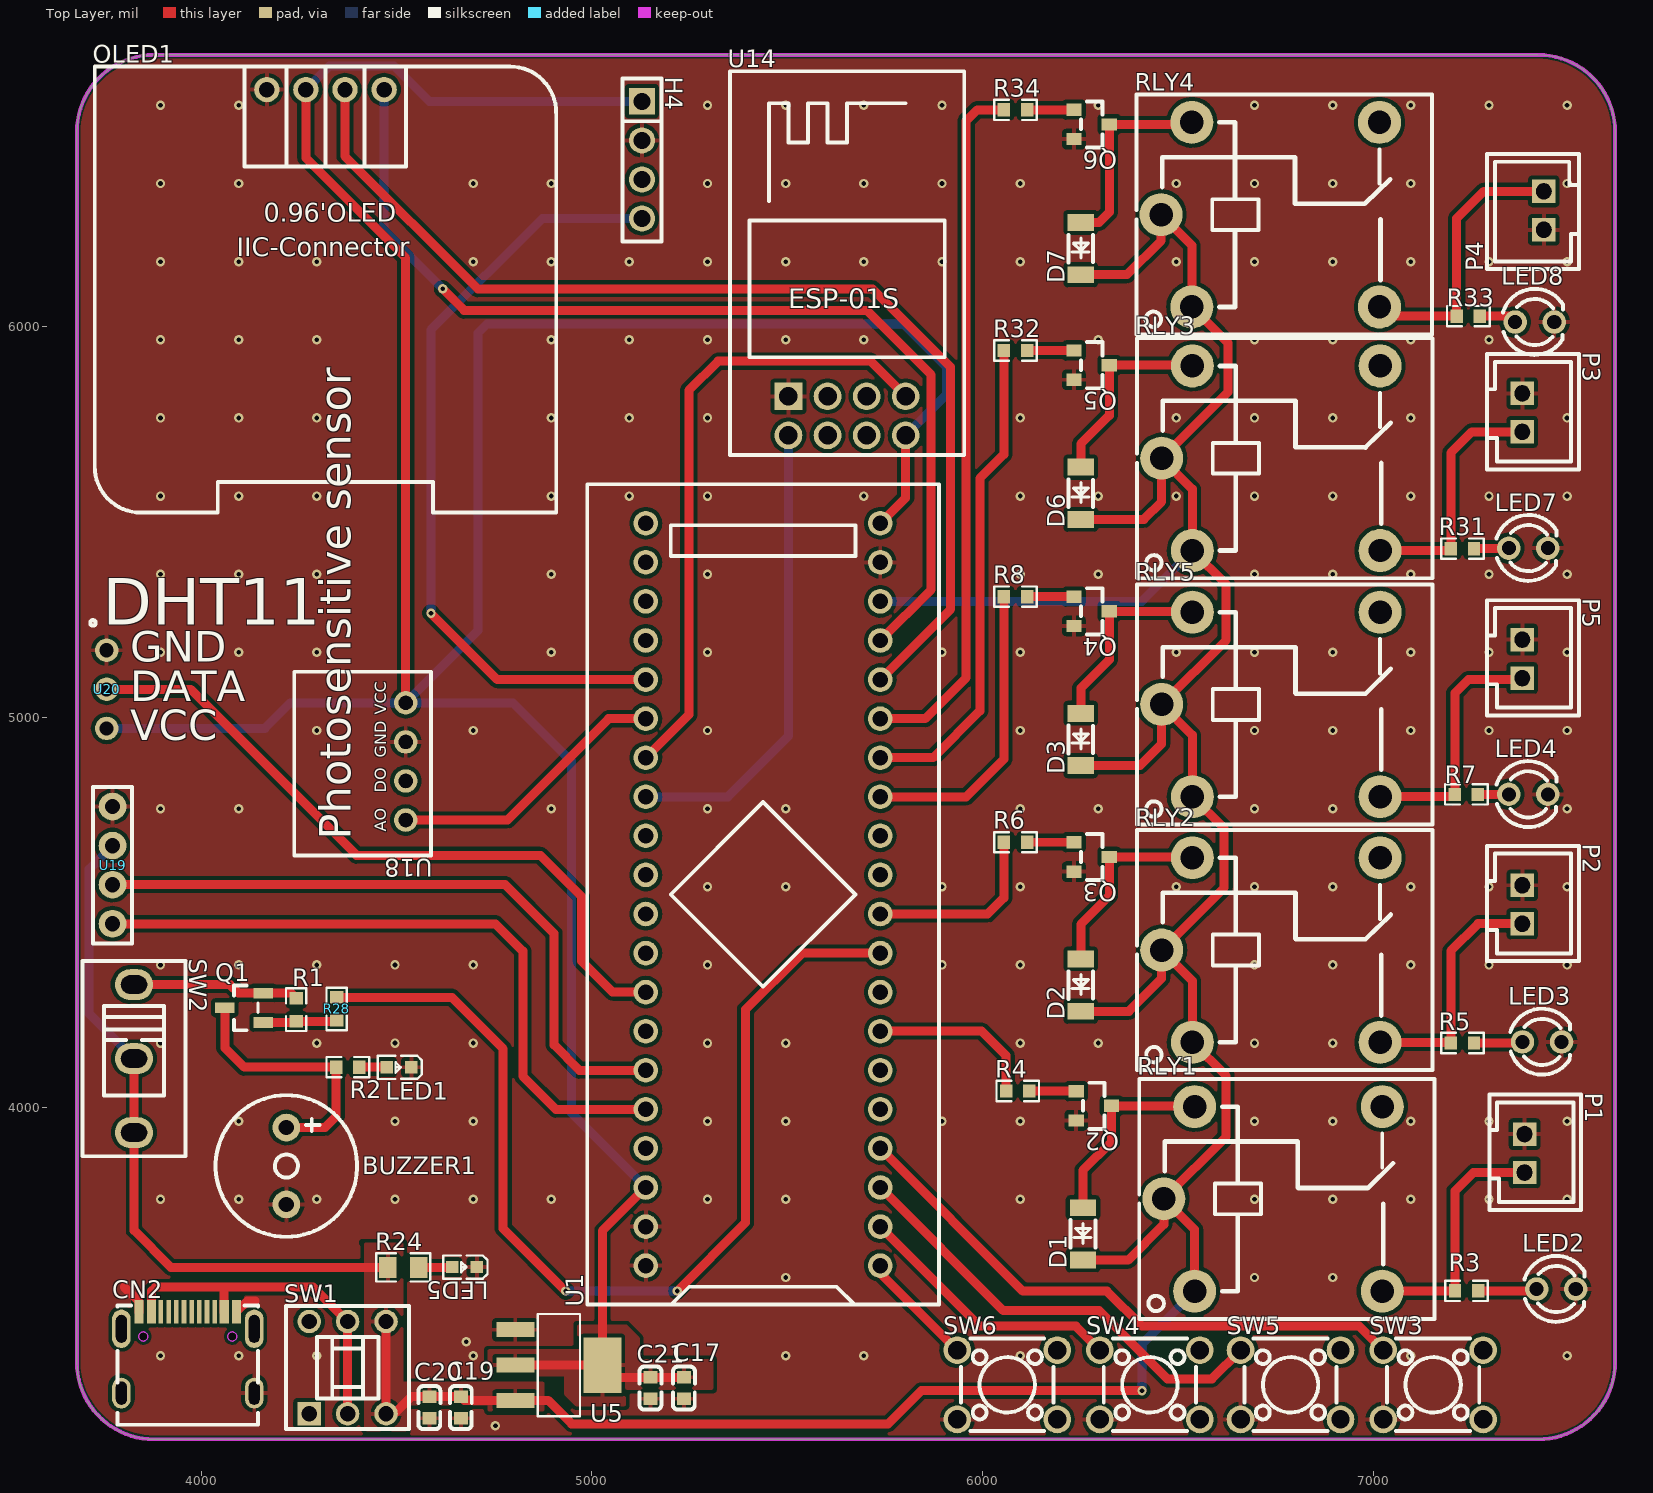
[diagram p0: Top Layer view]
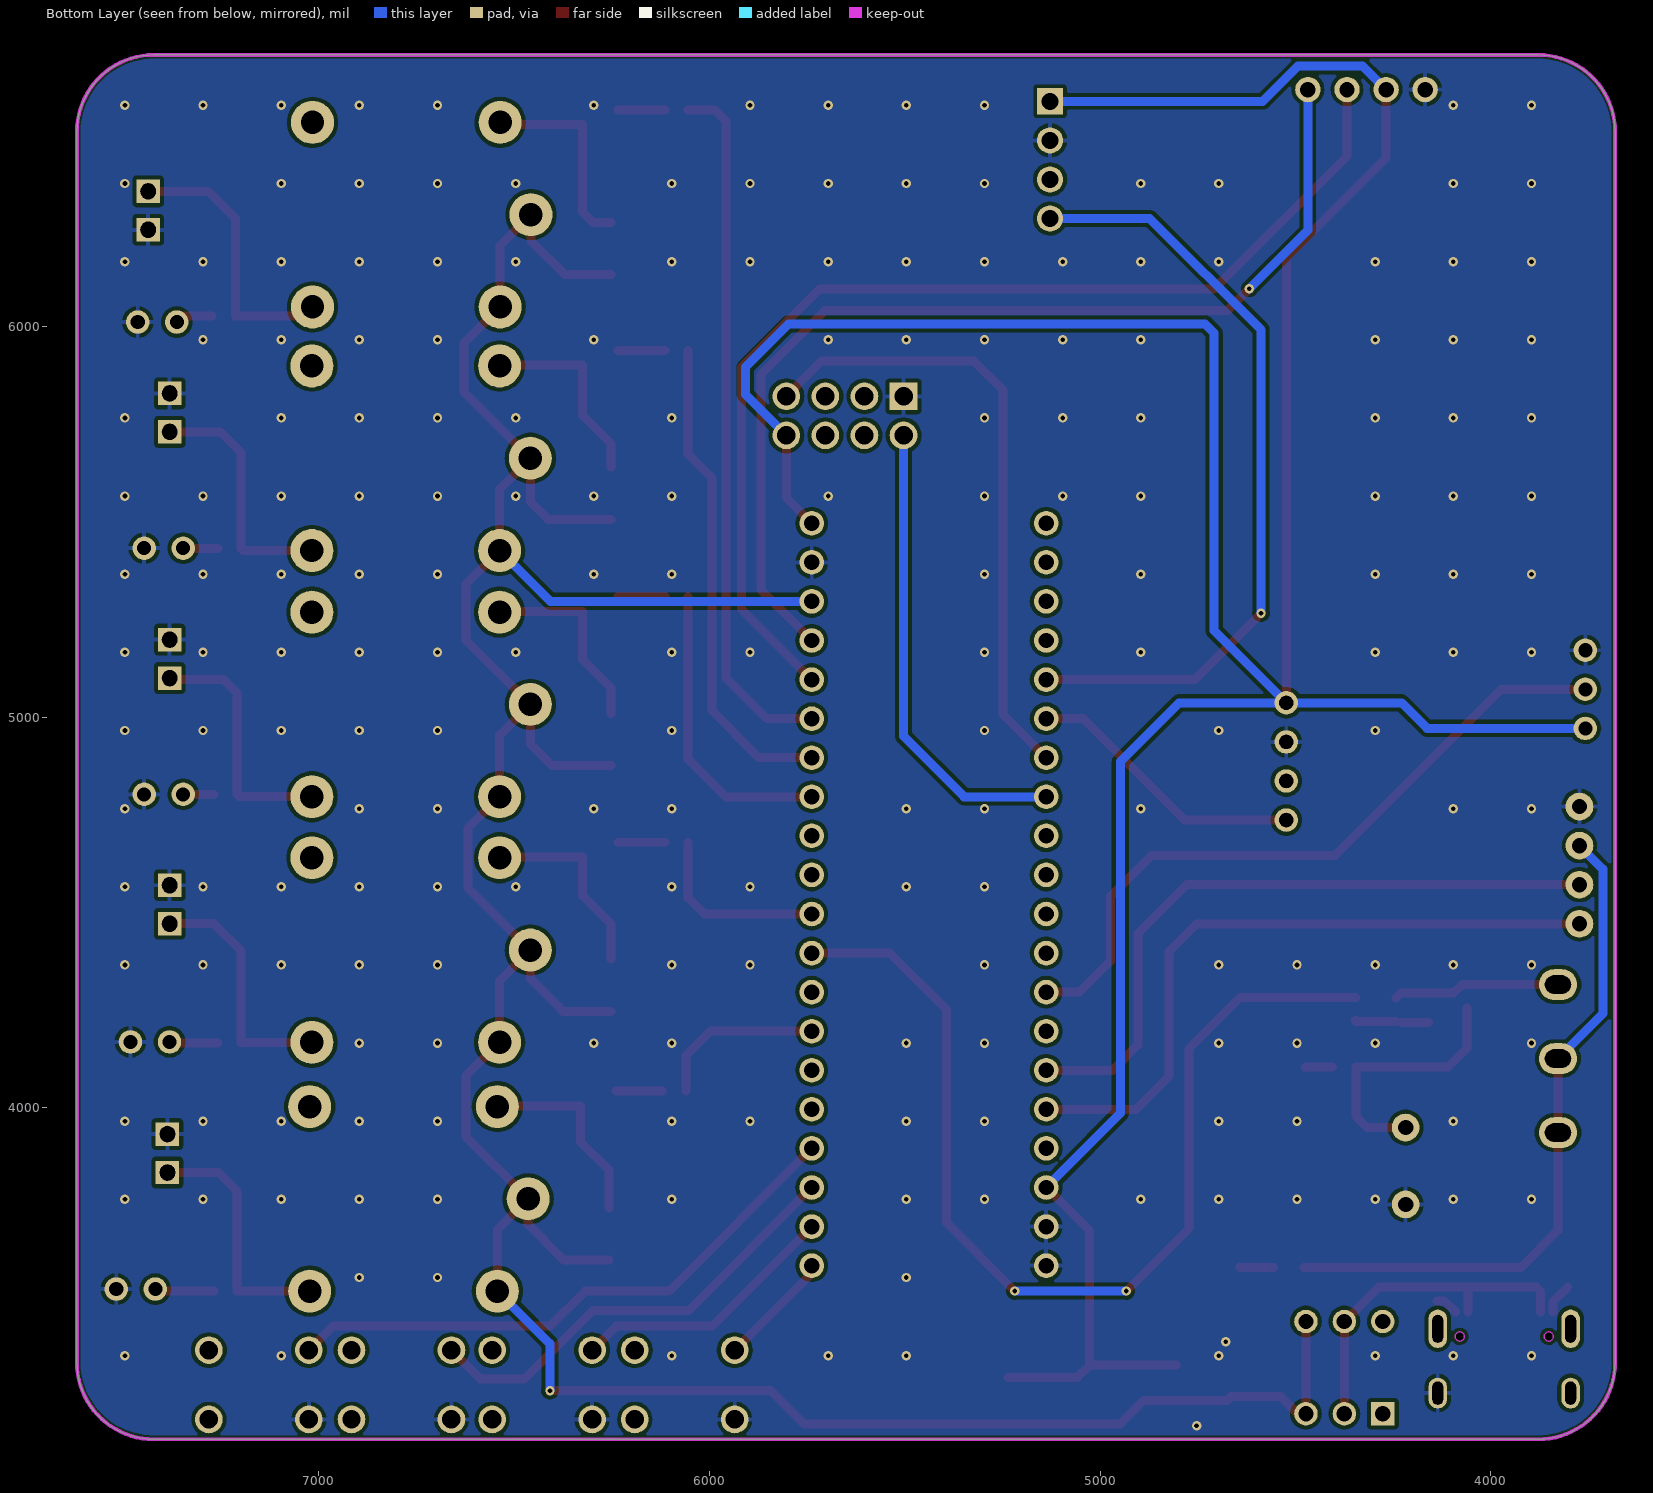
[diagram p1: Bottom Layer view, seen from below]
# Altium PCB MISC51965.pcbdoc
Units mil, origin at the board's own origin, x right, y up, seen from the top; angles counter-clockwise.
Board outline 3937.01 x 3543.31 mil, 2 copper layers (Top Layer, Bottom Layer), stack 62.206 mil thick; 62 components, 48 nets, 227 pads, 205 vias.

## Layer stack, top to bottom
Top Solder Mask Layer: solder mask 0.394, Dk 3.3
Top Layer: signal copper 1.379
Dielectric1: surface 59.449, FR4, Dk 4.5
Bottom Layer: signal copper 1.378
Bottom Solder Mask Layer: solder mask 0.394, Dk 3.3

## Board outline
3879.19,6694.72 ccw(c3879.19,6497.87) 3682.34,6497.87 3682.34,3348.26 ccw(c3879.19,3348.26) 3879.19,3151.41 7422.5,3151.41 ccw(c7422.5,3348.26) 7619.35,3348.26 7619.35,6497.87 ccw(c7422.5,6497.87) 7422.5,6694.72 3879.19,6694.72

## Design rules (kind name [scope] priority, off if disabled: settings)
BoardOutlineClearance copperThickness2oz_1 [All] p2 off: genericclearance=7.99 ignorepadtopadclearanceinfootprint=FALSE except(0: Arc-SplitContinuation Track-SplitContinuation SMDPad-SplitContinuation THPad-SplitContinuation Via-SplitContinuation Fill-SplitContinuation Region-SplitContinuation Poly-SplitContinuation Text-SplitContinuation Hole-SplitContinuation; 5.98: Arc-CutoutEdge SMDPad-CutoutEdge THPad-CutoutEdge Via-CutoutEdge Fill-CutoutEdge Region-CutoutEdge Text-CutoutEdge; 6.93: Hole-OutlineEdge Hole-CutoutEdge; 10: Poly-OutlineEdge Poly-CutoutEdge; 11.81: Arc-OutlineEdge Track-OutlineEdge SMDPad-OutlineEdge THPad-OutlineEdge Via-OutlineEdge Fill-OutlineEdge Region-OutlineEdge Text-OutlineEdge Track-CutoutEdge)
BoardOutlineClearance copperThickness1oz_1 [All] p4: genericclearance=4.02 ignorepadtopadclearanceinfootprint=FALSE except(0: Arc-SplitContinuation Track-SplitContinuation SMDPad-SplitContinuation THPad-SplitContinuation Via-SplitContinuation Fill-SplitContinuation Region-SplitContinuation Poly-SplitContinuation Text-SplitContinuation Hole-SplitContinuation; 6: SMDPad-CutoutEdge THPad-CutoutEdge Via-CutoutEdge Fill-CutoutEdge Region-CutoutEdge Text-CutoutEdge; 6.93: Hole-OutlineEdge Hole-CutoutEdge; 10: Poly-OutlineEdge Poly-CutoutEdge; 11.8: Arc-OutlineEdge Track-OutlineEdge SMDPad-OutlineEdge THPad-OutlineEdge Via-OutlineEdge Fill-OutlineEdge Region-OutlineEdge Text-OutlineEdge; 11.81: Arc-CutoutEdge Track-CutoutEdge)
Clearance copperThickness2oz [All] p1 off: gap=7.99 ignorepadtopadclearanceinfootprint=FALSE except(5.98: SMDPad-Track SMDPad-SMDPad THPad-Track SMDPad-THPad THPad-THPad Track-Via SMDPad-Via THPad-Via Via-Via Fill-Track Region-Track Fill-SMDPad Region-SMDPad Fill-THPad Region-THPad Fill-Via Region-Via Fill-Fill Fill-Region Region-Region Arc-Track Arc-SMDPad Arc-THPad Arc-Via Fill-Arc Region-Arc Arc-Arc Text-Track SMDPad-Text Text-THPad Text-Via Fill-Text Region-Text Arc-Text Text-Text; 6.93: Hole-Track Hole-SMDPad Hole-THPad Hole-Via Fill-Hole Region-Hole Hole-Arc Hole-Text; 10: Poly-Track Poly-SMDPad Poly-THPad Poly-Via Poly-Fill Poly-Region Poly-Poly Poly-Arc Poly-Text Poly-Hole)
Clearance copperThickness1oz [All] p3: gap=4.02 ignorepadtopadclearanceinfootprint=FALSE except(5.98: SMDPad-Track SMDPad-SMDPad THPad-Track SMDPad-THPad THPad-THPad Track-Via SMDPad-Via THPad-Via Via-Via Fill-Track Region-Track Fill-SMDPad Region-SMDPad Fill-THPad Region-THPad Fill-Via Region-Via Fill-Fill Fill-Region Region-Region; 6: Arc-Track Arc-SMDPad Arc-THPad Arc-Via Fill-Arc Region-Arc Arc-Arc Text-Track SMDPad-Text Text-THPad Text-Via Fill-Text Region-Text Arc-Text Text-Text; 6.93: Hole-Track Hole-SMDPad Hole-THPad Hole-Via Fill-Hole Region-Hole Hole-Arc Hole-Text; 10: Poly-Track Poly-SMDPad Poly-THPad Poly-Via Poly-Fill Poly-Region Poly-Poly Poly-Arc Poly-Text Poly-Hole)
DiffPairsRouting differentialPair [All] p1: maxlimit=6 minlimit=6 mostfreqgap=6 toplayer_minwidth=5 toplayer_prefwidth=10 toplayer_maxwidth=100 toplayer_mingap=6 toplayer_prefgap=6 toplayer_maxgap=6 bottomlayer_minwidth=5 bottomlayer_prefwidth=10 bottomlayer_maxwidth=100 bottomlayer_mingap=6 bottomlayer_prefgap=6 bottomlayer_maxgap=6 maxuncoupledlength=10
HoleToHoleClearance otherClearance [All] p1: gap=11.81 allowstackedmicrovias=TRUE
Length netLength [All] p1: minlimit=0 maxlimit=0
MatchedLengths netLengthTolerance [All] p1: tolerance=1000
PasteMaskExpansion pasteMaskExpansion [All] p1: expansion=0
PlaneConnect innerPlane [All] p1: planeconnectstyle=Relief reliefexpansion=20 reliefentries=4 reliefconductorwidth=10 reliefairgap=10
PolygonConnect copperRegion [All] p1: connectstyle=Relief reliefconductorwidth=10 reliefentries=4 polygonreliefangle="90 Angle" airgapwidth=10 via.connectstyle=Relief via.reliefconductorwidth=10 via.reliefentries=4 via.polygonreliefangle="90 Angle" via.airgapwidth=10
RoutingVias viaSize [All] p1: holewidth=12.01 width=24.02 viastyle="Through Hole" minholewidth=11.81 minwidth=19.68 maxholewidth=248.03 maxwidth=393.7
SolderMaskExpansion solderMaskExpansion [IsVia] p1: expansion=-1000 istentingtop=TRUE
SolderMaskExpansion solderMaskExpansion [All] p2: expansion=2 istentingtop=FALSE
Width copperThickness2oz_2 [All] p1 off: maxlimit=100 minlimit=8 preferedwidth=10
Width copperThickness1oz_2 [All] p2: maxlimit=100 minlimit=5 preferedwidth=10

## Components (designator, comment, footprint, x,y, rotation, side; value= is the part's Value field where it differs from the comment)
BUZZER1 "HNB09A03" BUZ-TH_BD9.0-P5.00-D0.6-FD 4218.56,3850.88 r270 top
C17 "100n" C0603 5236.12,3282.62 r90 top
C19 "100n" C0603 4665.04,3232.75 r90 top
C20 "10u" C0603 4584.63,3232.75 r90 top
C21 "22u" C0603 5150.42,3282.62 r90 top
CN2 "USB-TYPEC" USB-C-SMD_MC-307 3966.22,3373.55 r0 top
D1 "LL4148" LL-34_L3.5-W1.5-RD 6257.42,3676.99 r90 top
D2 "LL4148" LL-34_L3.5-W1.5-RD 6251.77,4313.8 r90 top
D3 "LL4148" LL-34_L3.5-W1.5-RD 6251.77,4942.46 r90 top
D6 "LL4148" LL-34_L3.5-W1.5-RD 6251.77,5572.56 r90 top
D7 "LL4148" LL-34_L3.5-W1.5-RD 6251.77,6198.97 r90 top
H4 "" HDR-TH_4P-P2.54-V-F 5128.56,6425.88 r270 top
LED1 "" LED_0603 4504.75,4103.27 r180 top
LED2 "" LED_TH-3mm 7468.56,3535.88 r0 top
LED3 "" LED_TH-3mm 7432.24,4168.48 r0 top
LED4 "" LED_TH-3mm 7397.24,4802.14 r0 top
LED5 "" LED_0603 4672.56,3592.05 r180 top
LED7 "" LED_TH-3mm 7397.24,5432.23 r0 top
LED8 "" LED_TH-3mm 7413.56,6010.88 r0 top
OLED1 "" 0.96OLED_4P 4318.56,6605.88 r0 top
P1 "XH2.54 straight socket 2P" CONN-TH_XH2.54-2P 7387.52,3883.4 r270 top
P2 "XH2.54 straight socket 2P" CONN-TH_XH2.54-2P 7381.88,4520.21 r270 top
P3 "XH2.54 straight socket 2P" CONN-TH_XH2.54-2P 7381.88,5778.97 r270 top
P4 "XH2.54 straight socket 2P" CONN-TH_XH2.54-2P 7436.88,6296.23 r90 top
P5 "XH2.54 straight socket 2P" CONN-TH_XH2.54-2P 7381.88,5148.87 r270 top
Q1 "" S8550P_SOT 4108.56,4255.88 r0 top
Q2 "" S8050_SOT-23 6285.17,4009.98 r180 top
Q3 "" S8050_SOT-23 6279.53,4646.79 r180 top
Q4 "" S8050_SOT-23 6279.53,5275.45 r180 top
Q5 "" S8050_SOT-23 6279.53,5905.55 r180 top
Q6 "" S8050_SOT-23 6279.53,6521.7 r180 top
R1 "10k" R0603 4243.56,4250.88 r270 top
R2 "1k" R0603 4375.75,4103.67 r180 top
R3 "3.3k" R0603 7239.24,3531.48 r0 top
R4 "1k" R0603 6090.38,4042.7 r0 top
R5 "3.3k" R0603 7228.56,4165.88 r0 top
R6 "1k" R0603 6084.73,4679.51 r0 top
R7 "3.3k" R0603 7238.6,4801.95 r0 top
R8 "1k" R0603 6084.73,5308.17 r0 top
R24 "4.7k" R0805 4517.71,3591.37 r0 top
R28 "1k" R0603 4347.14,4252.97 r270 top
R31 "3.3k" R0603 7228.56,5430.88 r0 top
R32 "1k" R0603 6084.73,5938.26 r0 top
R33 "3.3k" R0603 7243.56,6025.88 r0 top
R34 "1k" R0603 6084.73,6554.14 r0 top
RLY1 "SRD-05VDC-SL-C" RELAY-TH_SRD-XXVDC-XL-C 6743.86,3766.8 r0 top
RLY2 "SRD-05VDC-SL-C" RELAY-TH_SRD-XXVDC-XL-C 6738.22,4403.6 r0 top
RLY3 "SRD-05VDC-SL-C" RELAY-TH_SRD-XXVDC-XL-C 6738.22,5662.36 r0 top
RLY4 "SRD-05VDC-SL-C" RELAY-TH_SRD-XXVDC-XL-C 6736.75,6285.76 r0 top
RLY5 "SRD-05VDC-SL-C" RELAY-TH_SRD-XXVDC-XL-C 6738.22,5032.27 r0 top
SW1 "K8-8081D-NNW" SW-TH_6P-L8.0-W8.0-P2.50 4375.18,3334.76 r0 top
SW2 "XY-SS12D10L3" SW-TH_3P-L12.7-W6.7_XY-SS12D10LXX 3828.56,4125.88 r270 top
SW3 "" SW-TH_4P-L6.0-W6.0-P4.50-LS6.5 7153.56,3290.88 r0 top
SW4 "" SW-TH_4P-L6.0-W6.0-P4.50-LS6.5 6428.56,3290.88 r0 top
SW5 "" SW-TH_4P-L6.0-W6.0-P4.50-LS6.5 6788.56,3290.88 r0 top
SW6 "" SW-TH_4P-L6.0-W6.0-P4.50-LS6.5 6063.56,3290.88 r0 top
U1 "LCKFB-DKX-STM32F103C8T6" CONN-TH_L53.3-W22.9_STM32F103C8T6-CARD 5438.56,4545.88 r90 top
U5 "TLV1117LV33DCYT" SOT-223-4_L6.5-W3.5-P2.30-LS7.0-BR 4915.99,3341.32 r180 top
U14 "ESP-01S" WIFIM-TH_ESP-01S 5653.56,5770.88 r0 top
U18 "Light intensity module" 光敏传感器 4498.56,4870.88 r180 top
U19 "" 4P排母 3723.56,4820.88 r270 top
U20 "" dht11温湿度传感器 3758.56,5170.88 r0 top

## Footprints (in the part's own frame and the unit in brackets; to place one, negate y for a bottom-side part, rotate by r counter-clockwise, add the part's x,y. Pads: shape width x height; smd on the part's side, far side on the other; paste and mask are expansions set on the pad)
0.96OLED_4P [mm]
  round 1.65 hole 1 copper offset 0,0: 1(-3.81,-0.001) 2(-1.27,0.002) 3(1.27,0.002) 4(3.81,0.002)
  silkscreen extent -15,-27.5 15,1.5
4P排母 [mm]
  round 1.8 hole 1: 1(1.27,1.27) 2(3.81,1.27) 3(6.35,1.27) 4(8.89,1.27)
  silkscreen extent 0,0 10.16,2.54
BUZ-TH_BD9.0-P5.00-D0.6-FD [mm]
  round 1.8 hole 1 copper offset 0,0 paste+0 mask+0.051: 1(-2.5,0) 2(2.5,0)
  silkscreen extent -4.6,-4.6 4.6,4.6
C0603 [mm]
  rect 0.8x0.9 smd paste+0 mask+0.051: 1(-0.7,0) 2(0.7,0)
  silkscreen extent -1.41,-0.71 1.39,0.72
CONN-TH_L53.3-W22.9_STM32F103C8T6-CARD [mm]
  round 1.6 hole 1: 1(-24.13,-7.62) 2(-21.59,-7.62) 3(-19.05,-7.62) 4(-16.51,-7.62) 5(-13.97,-7.62) 6(-11.43,-7.62) 7(-8.89,-7.62) 8(-6.35,-7.62) 9(-3.81,-7.62) 10(-1.27,-7.62) 11(1.27,-7.62) 12(3.81,-7.62) 13(6.35,-7.62) 14(8.89,-7.62) 15(11.43,-7.62) 16(13.97,-7.62) 17(16.51,-7.62) 18(19.05,-7.62) 19(21.59,-7.62) 20(24.13,-7.62) 21(24.13,7.62) 22(21.59,7.62) 23(19.05,7.62) 24(16.51,7.62) 25(13.97,7.62) 26(11.43,7.62) 27(8.89,7.62) 28(6.35,7.62) 29(3.81,7.62) 30(1.27,7.62) 31(-1.27,7.62) 32(-3.81,7.62) 33(-6.35,7.62) 34(-8.89,7.62) 35(-11.43,7.62) 36(-13.97,7.62) 37(-16.51,7.62) 38(-19.05,7.62) 39(-21.59,7.62) 40(-24.13,7.62)
  silkscreen extent -26.67,-11.43 26.67,11.43
CONN-TH_XH2.54-2P [mil]
  rect 60x60 hole 39.37 slot 41.34 at 0 deg paste+0 mask+1.97: 1(-49.22,0) 2(49.21,0)
  silkscreen extent -150,-90 145,145
dht11温湿度传感器 [mil]
  round 60 hole 36: 1(0,0) 2(0,-100) 3(0,-200)
  silkscreen extent -42,63 -28,77
HDR-TH_4P-P2.54-V-F [mm]
  rect 1.7x1.7 hole 1.1: 1(-3.81,0)
  round 1.7 hole 1.1: 2(-1.27,0) 3(1.27,0) 4(3.81,0)
  silkscreen extent -5.29,-1.27 5.29,1.27
LED_0603 [mil]
  rect 31.5x31.5 smd paste+0 mask+2: 1(-33.5,-0.4) 2(29.5,-0.2)
  silkscreen extent -61,-30 53,30
LED_TH-3mm [mil]
  round 60 hole 36 paste+0 mask+2: 1(-50,0) 2(50,0)
  silkscreen extent -81,-84 72,85
LL-34_L3.5-W1.5-RD [mm]
  rect 1.1x1.7 smd paste+0 mask+0.051: 1(-1.7,0) 2(1.7,0)
  silkscreen extent -0.9,-0.8 0.9,0.8
R0603 [mil]
  rect 31.75x34.02 smd paste-3937.01 mask+2: 1(-29.65,0) 2(29.66,0)
  silkscreen extent -55,-26 55,26
R0805 [mm]
  rect 1.133x1.377 smd paste-100 mask+0.051: 1(-1,0) 2(1,0)
  silkscreen extent -1.76,-0.92 1.76,0.92
RELAY-TH_SRD-XXVDC-XL-C [mil]
  round 110 hole 60: 1(-200.79,-236.22) 2(279.53,-236.2) 3(279.53,236.2) 4(-200.79,236.22) 5(-279.53,0)
  silkscreen extent -342,-307 413,307
S8050_SOT-23 [mm]
  rect 1x0.8 smd paste+0 mask+0.051: 1(1.15,-0.823) 2(1.15,1.077) 3(-1.15,0.127)
  silkscreen extent -0.7,-1.37 0.7,1.63
S8550P_SOT [mil]
  rect 49.2x27.6 smd paste+0 mask+2: 1(50.84,-37.4) 2(50.84,37.4) 3(-47.56,0)
  silkscreen extent -24,-58 37,58
SOT-223-4_L6.5-W3.5-P2.30-LS7.0-BR [mm]
  rect 2.47x0.98 smd paste+0 mask+0.051: 1(2.835,-2.3) 2(2.835,0) 3(2.835,2.3)
  rect 2.47x3.6 smd paste+0 mask+0.051: 4(-2.835,0)
  silkscreen extent -1.37,-3.33 1.37,3.33
SW-TH_3P-L12.7-W6.7_XY-SS12D10LXX [mm]
  oval 2x2.5 hole 1.2 slot 1.7 at 90 deg: 1(-4.81,0) 2(0,0) 3(4.81,0)
  silkscreen extent -6.35,-3.35 6.35,3.35
SW-TH_4P-L6.0-W6.0-P4.50-LS6.5 [mm]
  round 1.8 hole 1.2: 1(-3.25,2.25) 2(3.25,2.25) 3(-3.25,-2.25) 4(3.25,-2.25)
  silkscreen extent -3,-3 3,3
SW-TH_6P-L8.0-W8.0-P2.50 [mil]
  rect 60x60 hole 39.37 paste+0 mask+2: 1(-98.43,-118.11)
  round 60 hole 39.37 paste+0 mask+2: 2(0,-118.11) 3(98.42,-118.11) 4(-98.43,118.11) 5(0,118.11) 6(98.42,118.11)
  silkscreen extent -157,-157 157,157
USB-C-SMD_MC-307 [mm]
  oval 1.2x2 hole 0.7 slot 1.5 at 90 deg paste+0 mask+0.051: 0(4.32,-2.64) 1(-4.32,-2.64)
  oval 1.2x2.5 hole 0.7 slot 1.8 at 90 deg paste+0 mask+0.051: 2(4.32,1.54) 3(-4.32,1.54)
  rect 0.6x1.524 smd paste-100 mask+0.051: A1B12(-3.165,2.64) A4B9(-2.365,2.64) B1A12(3.165,2.64) B4A9(2.365,2.64)
  rect 0.3x1.524 smd paste-100 mask+0.051: A5(-1.25,2.64) A6(-0.25,2.64) A7(0.25,2.64) A8(1.25,2.64) B5(1.75,2.64) B6(0.75,2.64) B7(-0.75,2.64) B8(-1.75,2.64)
  Board Outline Layer circle w0.003: c-2.89,1.04 r0.3
  Board Outline Layer circle w0.003: c2.89,1.04 r0.3
  Board Outline Layer region: -2.59,1.04 -2.62,0.91 -2.703,0.806 -2.823,0.748 -2.957,0.748 -3.077,0.806 -3.16,0.91 -3.19,1.04 -3.19,1.04 -3.16,1.17 -3.077,1.275 -2.957,1.333 -2.823,1.333 -2.703,1.275 -2.62,1.17 -2.59,1.04
  Board Outline Layer region: -2.59,1.04 -2.599,0.968 -2.624,0.901 -2.665,0.841 -2.72,0.793 -2.784,0.76 -2.854,0.742 -2.926,0.742 -2.996,0.76 -3.06,0.793 -3.115,0.841 -3.156,0.901 -3.181,0.968 -3.19,1.04 -3.181,1.112 -3.156,1.18 -3.115,1.239 -3.06,1.287 -2.996,1.321 -2.926,1.338 -2.854,1.338 -2.784,1.321 -2.72,1.287 -2.665,1.239 -2.624,1.18 -2.599,1.112
  Board Outline Layer region: 3.19,1.04 3.16,0.91 3.077,0.806 2.957,0.748 2.823,0.748 2.703,0.806 2.62,0.91 2.59,1.04 2.59,1.04 2.62,1.17 2.703,1.275 2.823,1.333 2.957,1.333 3.077,1.275 3.16,1.17 3.19,1.04
  Board Outline Layer region: 3.19,1.04 3.181,0.968 3.156,0.901 3.115,0.841 3.06,0.793 2.996,0.76 2.926,0.742 2.854,0.742 2.784,0.76 2.72,0.793 2.665,0.841 2.624,0.901 2.599,0.968 2.59,1.04 2.599,1.112 2.624,1.18 2.665,1.239 2.72,1.287 2.784,1.321 2.854,1.338 2.926,1.338 2.996,1.321 3.06,1.287 3.115,1.239 3.156,1.18 3.181,1.112
  Multi-Layer board cut-out: -2.59,1.04 -2.62,0.91 -2.703,0.806 -2.823,0.748 -2.957,0.748 -3.077,0.806 -3.16,0.91 -3.19,1.04 -3.19,1.04 -3.16,1.17 -3.077,1.275 -2.957,1.333 -2.823,1.333 -2.703,1.275 -2.62,1.17 -2.59,1.04
  Multi-Layer board cut-out: 3.19,1.04 3.16,0.91 3.077,0.806 2.957,0.748 2.823,0.748 2.703,0.806 2.62,0.91 2.59,1.04 2.59,1.04 2.62,1.17 2.703,1.275 2.823,1.333 2.957,1.333 3.077,1.275 3.16,1.17 3.19,1.04
  silkscreen extent -4.57,-4.7 4.57,3.05
WIFIM-TH_ESP-01S [mm]
  rect 1.8x1.8 hole 1.2: 1(-3.81,1.27)
  round 1.8 hole 1.2: 2(-1.27,1.27) 3(1.27,1.27) 4(3.81,1.27) 5(3.81,-1.27) 6(1.27,-1.27) 7(-1.27,-1.27) 8(-3.81,-1.27)
  silkscreen extent -7.62,-2.54 7.62,22.4
光敏传感器 [mil]
  round 60 hole 36 slot 36.2 at 90 deg: 1(-25.45,-165.45) 2(-25.45,-65.45) 3(-25.45,34.55) 4(-25.45,134.55)
  silkscreen extent -90,-245 260,225

## Via types
v1: diameter 24.02, hole 12, Top Layer to Bottom Layer, 205 vias

## Nets (pads, with @x,y where several pads share a name; then routed paths per layer and width w, separated by ;. In a path a pad name is that pad's centre, name@x,y a point inside that pad or via, vN(x,y) a via of type N, cw(c..) or ccw(c..) an arc to the next point about the centre after c; other vN are vias at no path point)
$1N25: Q6.1 R34.2 | length 119.8
  Top Layer w23: R34.2 Q6.1@6234.21,6554.14
$1N27: D7.2 Q6.3 RLY4.4 | length 521.8
  Top Layer w23: D7.2 6298.58,6265.9 6324.8,6292.12 Q6.3 6530.68,6516.7 RLY4.4
$1N29: P4.2 R33.1 RLY4.2 | length 709.4
  Top Layer w23: RLY4.2 7039.96,6025.88 R33.1 7213.9,6276.22 7283.13,6345.45 P4.2
$1N33: LED8.1 R33.2 | length 96.6
  Top Layer w23: R33.2 7348.56,6025.88 LED8.1
$1N35: Q5.1 R32.2 | length 120
  Top Layer w23: R32.2 6233.94,5938.26 Q5.1
$1N37: D6.2 Q5.3 RLY3.4 | length 504.7
  Top Layer w23: D6.2 6251.77,5699.09 6324.8,5772.12 Q5.3 6535.46,5900.54 RLY3.4
$1N39: P3.2 R31.1 RLY3.2 | length 633.6
  Top Layer w23: RLY3.2 7194.18,5426.16 R31.1 7198.9,5676.22 7252.43,5729.75 P3.2
$1N43: LED7.1 R31.2 | length 89.6
  Top Layer w23: R31.2 7345.89,5430.88 LED7.1
$1N57: LED5.2 R24.2 | length 86.3
  Top Layer w23: R24.2 4642.18,3591.37 LED5.2
$1N74: BUZZER1.1 Q1.3 R2.2 | length 673
  Top Layer w23: Q1.3 4061,4153.44 4110.77,4103.67 R2.2 4346.09,3978.41 4316.98,3949.3 BUZZER1.1
$1N76: Q1.1 R1.2 R28.2 | length 173.6
  Top Layer w23: Q1.1 R1.2@4228.56,4218.48 ; R1.2 4345.05,4221.22 R28.2
$1N136: Q1.2 R1.1 SW2.1 | length 429.4
  Top Layer w23: SW2.1@3828.56,4315.25 4074.19,4315.25 4096.16,4293.28 Q1.2 4230.81,4293.28 R1.1
$1N137: LED1.2 R2.1 | length 69.9
  Top Layer w23: R2.1 4475.05,4103.67 LED1.2
$1N147: Q2.1 R4.2 | length 120
  Top Layer w23: R4.2 6239.58,4042.7 Q2.1
$1N149: D1.2 Q2.3 RLY1.4 | length 504.7
  Top Layer w23: D1.2 6257.42,3839.74 6330.45,3912.77 Q2.3 6541.11,4004.98 RLY1.4
$1N151: P1.2 R3.1 RLY1.2 | length 639.5
  Top Layer w23: RLY1.2 7208.7,3530.6 R3.1 7209.58,3786.9 7256.87,3834.19 P1.2
$1N155: LED2.1 R3.2 | length 151.5
  Top Layer w23: R3.2 7414.16,3531.48 LED2.1
$1N157: Q3.1 R6.2 | length 120
  Top Layer w23: R6.2 6233.94,4679.51 Q3.1
$1N159: D2.2 Q3.3 RLY2.4 | length 504.7
  Top Layer w23: D2.2 6251.77,4469.09 6324.8,4542.12 Q3.3 6535.46,4641.79 RLY2.4
$1N161: P2.2 R5.1 RLY2.2 | length 629
  Top Layer w23: RLY2.2 7197.37,4167.4 R5.1 7198.9,4401.22 7268.68,4470.99 P2.2
$1N165: LED3.1 R5.2 | length 125.1
  Top Layer w23: R5.2 7379.64,4165.88 LED3.1
$1N170: Q4.1 R8.2 | length 120
  Top Layer w23: R8.2 6233.94,5308.17 Q4.1
$1N172: D3.2 Q4.3 RLY5.4 | length 504.7
  Top Layer w23: D3.2 6251.77,5074.09 6324.8,5147.12 Q4.3 6535.46,5270.45 RLY5.4
$1N174: P5.2 R7.1 RLY5.2 | length 641.8
  Top Layer w23: RLY5.2 7203.06,4796.07 R7.1 7208.94,5061.26 7243.56,5095.88 7378.1,5095.88 P5.2
$1N178: LED4.1 R7.2 | length 79.1
  Top Layer w23: R7.2 7347.05,4801.95 LED4.1
+5V: C19.2 C20.2 D1.1 D2.1 D3.1 D6.1 D7.1 R24.1 RLY1.1 RLY1.5 RLY2.1 RLY2.5 RLY3.1 RLY3.5 RLY4.1 RLY4.5 RLY5.1 RLY5.5 SW1.3 SW1.6 SW2.2 SW2.3 U1.18 U5.3 U19.2 | length 10095.8
  Top Layer w23: SW2.2 SW2.3 3828.56,3685.88 3923.07,3591.37 R24.1 ; SW1.6 SW1.3 4494.33,3216.65 4537.99,3260.31 C20.2 C19.2 4674.58,3250.77 U5.3 4888.66,3250.77 4948.56,3190.88 5758.56,3190.88 5843.56,3275.88 v1(6408.56,3275.88) ; D2.1 6374.55,4246.87 6458.69,4331.01 RLY2.5 ; D3.1 6403.21,4875.53 6458.69,4931.01 RLY5.5 ; D6.1 6413.31,5505.63 6458.69,5551.01 RLY3.5 ; D7.1 6369.72,6132.03 6457.22,6219.54 RLY4.5 6535.96,6207.02 RLY4.1 6628.56,5956.94 6628.56,5832.23 RLY3.5 ; D1.1 6372.74,3610.06 6464.33,3701.65 RLY1.5 ; RLY1.1 6543.07,3688.06 RLY1.5 ; RLY2.5 6618.56,4563.47 6618.56,4714.92 RLY5.1 6537.43,4953.53 RLY5.5 ; RLY2.5 6537.43,4324.86 RLY2.1 6623.56,4081.25 6623.56,3926.02 RLY1.5 ; RLY5.5 6623.56,5197.13 6623.56,5340.01 RLY3.1 6537.43,5583.62 RLY3.5
  Bottom Layer w23: U19.2 3713.56,4610.88 3713.56,4240.88 SW2.2 ; U1.18 6407.17,5295.88 RLY3.1 ; v1(6408.56,3275.88) 6408.56,3396.06 RLY1.1
BEEP: R28.1 U1.9 | length 2649.8
  Top Layer w23: R28.1 4641.81,4282.62 4773.56,4150.88 4773.56,3690.88 v1(4933.56,3530.88) ; v1(5218.56,3530.88) 5393.56,3705.88 5393.56,4250.88 5538.56,4395.88 U1.9
  Bottom Layer w23: v1(4933.56,3530.88) v1(5218.56,3530.88)
ESP_RX: U1.27 U14.4 | length 1608.9
  Top Layer w23: U1.27 5248.56,5005.88 5248.56,5835.88 5323.56,5910.88 5713.56,5910.88 U14.4
ESP_TX: U1.28 U14.8 | length 1199.2
  Bottom Layer w23: U1.28 5348.56,4795.88 5503.56,4950.88 U14.8
GND: BUZZER1.2 C17.1 C19.1 C20.1 C21.1 CN2.0 CN2.A1B12 CN2.B1A12 H4.2 LED1.1 LED2.2 LED3.2 LED4.2 LED5.1 LED7.2 LED8.2 OLED1.1 P1.1 P2.1 P3.1 P4.1 P5.1 Q2.2 Q3.2 Q4.2 Q5.2 Q6.2 SW3.3 SW4.3 SW5.3 SW6.3 U1.19 U1.39 U1.40 U5.1 U14.1 U18.2 U19.1 U20.1 | length 138.7
  Top Layer w23: 3803.56,3540.88 3841.61,3502.83 CN2.A1B12 ; CN2.B1A12 4119.21,3505.88 4138.56,3505.88
  other v1: 4753.56,3185.88 3896.44,3365.51 4096.44,3365.51 4296.44,3365.51 4696.44,3365.51 5496.44,3365.51 5696.44,3365.51 6096.44,3365.51 7096.44,3365.51 7496.44,3365.51 4678.56,3400.88 5496.44,3565.51 6696.44,3565.51 6896.44,3565.51 3896.44,3765.51 4096.44,3765.51 4296.44,3765.51 4496.44,3765.51 4696.44,3765.51 4896.44,3765.51 5296.44,3765.51 5496.44,3765.51 6096.44,3765.51 6696.44,3765.51 6896.44,3765.51 7096.44,3765.51 7296.44,3765.51 7496.44,3765.51 4096.44,3965.51 4496.44,3965.51 4696.44,3965.51 5296.44,3965.51 5496.44,3965.51 5896.44,3965.51 6096.44,3965.51 6696.44,3965.51 6896.44,3965.51 7096.44,3965.51 7296.44,3965.51 7496.44,3965.51 3896.44,4165.51 4296.44,4165.51 4496.44,4165.51 4696.44,4165.51 5296.44,4165.51 5496.44,4165.51 6096.44,4165.51 6296.44,4165.51 6696.44,4165.51 6896.44,4165.51 3896.44,4365.51 4096.44,4365.51 4296.44,4365.51 4496.44,4365.51 4696.44,4365.51 5296.44,4365.51 5896.44,4365.51 6096.44,4365.51 6696.44,4365.51 6896.44,4365.51 7096.44,4365.51 7296.44,4365.51 7496.44,4365.51 5296.44,4565.51 5496.44,4565.51 5896.44,4565.51 6096.44,4565.51 6496.44,4565.51 6696.44,4565.51 6896.44,4565.51 7096.44,4565.51 7296.44,4565.51 7496.44,4565.51 3896.44,4765.51 4096.44,4765.51 4896.44,4765.51 5296.44,4765.51 5496.44,4765.51 6096.44,4765.51 6296.44,4765.51 6696.44,4765.51 6896.44,4765.51 7496.44,4765.51 4296.44,4965.51 4696.44,4965.51 5296.44,4965.51 6096.44,4965.51 6696.44,4965.51 6896.44,4965.51 7096.44,4965.51 7296.44,4965.51 7496.44,4965.51 3896.44,5165.51 4096.44,5165.51 4296.44,5165.51 4896.44,5165.51 5296.44,5165.51 5896.44,5165.51 6096.44,5165.51 6496.44,5165.51 6696.44,5165.51 6896.44,5165.51 7096.44,5165.51 7296.44,5165.51 7496.44,5165.51 3896.44,5365.51 4096.44,5365.51 4296.44,5365.51 4896.44,5365.51 5296.44,5365.51 6096.44,5365.51 6296.44,5365.51 6696.44,5365.51 6896.44,5365.51 7096.44,5365.51 7296.44,5365.51 7496.44,5365.51 3896.44,5565.51 4096.44,5565.51 4296.44,5565.51 4896.44,5565.51 5096.44,5565.51 5296.44,5565.51 5696.44,5565.51 6096.44,5565.51 6296.44,5565.51 6496.44,5565.51 6696.44,5565.51 6896.44,5565.51 7096.44,5565.51 7296.44,5565.51 7496.44,5565.51 3896.44,5765.51 4096.44,5765.51 4296.44,5765.51 4896.44,5765.51 5096.44,5765.51 5296.44,5765.51 6096.44,5765.51 6496.44,5765.51 6696.44,5765.51 6896.44,5765.51 7096.44,5765.51 7496.44,5765.51 3896.44,5965.51 4096.44,5965.51 4296.44,5965.51 4896.44,5965.51 5096.44,5965.51 5296.44,5965.51 5496.44,5965.51 5696.44,5965.51 6296.44,5965.51 6696.44,5965.51 6896.44,5965.51 7096.44,5965.51 7296.44,5965.51 3896.44,6165.51 4096.44,6165.51 4296.44,6165.51 4696.44,6165.51 4896.44,6165.51 5096.44,6165.51 5296.44,6165.51 5496.44,6165.51 5696.44,6165.51 5896.44,6165.51 6096.44,6165.51 6496.44,6165.51 6696.44,6165.51 6896.44,6165.51 7096.44,6165.51 7296.44,6165.51 7496.44,6165.51 3896.44,6365.51 4096.44,6365.51 4696.44,6365.51 4896.44,6365.51 5296.44,6365.51 5496.44,6365.51 5696.44,6365.51 5896.44,6365.51 6096.44,6365.51 6496.44,6365.51 6696.44,6365.51 6896.44,6365.51 7096.44,6365.51 7496.44,6365.51 3896.44,6565.51 4096.44,6565.51 5296.44,6565.51 5496.44,6565.51 5696.44,6565.51 5896.44,6565.51 6296.44,6565.51 6696.44,6565.51 6896.44,6565.51 7096.44,6565.51 7296.44,6565.51 7496.44,6565.51
JDQ1: R32.1 U1.14 | length 1252.6
  Top Layer w23: U1.14 5873.56,4895.88 5993.56,5015.88 5993.56,5610.88 6055.07,5672.39 R32.1
JDQ2: R34.1 U1.15 | length 1796.7
  Top Layer w23: U1.15 5853.56,4995.88 5958.56,5100.88 5958.56,6525.88 5986.82,6554.14 R34.1
JDQ3: R4.1 U1.7 | length 438.6
  Top Layer w23: U1.7 5998,4195.88 6060.72,4133.16 R4.1
JDQ4: R8.1 U1.13 | length 772.3
  Top Layer w23: U1.13 5958.56,4795.88 6055.07,4892.39 R8.1
JDQ5: R6.1 U1.10 | length 475.8
  Top Layer w23: U1.10 6013.56,4495.88 6055.07,4537.39 R6.1
KEY1: SW3.1 U1.4 | length 1501
  Top Layer w23: U1.4 6103.56,3530.88 6318.56,3530.88 6408.56,3440.88 6964.19,3440.88 SW3.1
KEY2: SW5.1 U1.3 | length 1155.5
  Top Layer w23: U1.3 6053.56,3480.88 6298.56,3480.88 6473.56,3305.88 6587.03,3305.88 SW5.1
KEY3: SW4.1 U1.2 | length 693.1
  Top Layer w23: U1.2 5993.56,3440.88 6239.19,3440.88 SW4.1
KEY4: SW6.1 U1.1 | length 298
  Top Layer w23: U1.1 5738.56,3576.51 SW6.1
PA0: H4.4 U1.25 | length 2003.5
  Top Layer w23: v1(4588.56,5265.88) 4758.56,5095.88 U1.25
  Bottom Layer w23: v1(4588.56,5265.88) 4588.56,5990.88 4873.56,6275.88 H4.4
PA1: U1.26 U18.4 | length 722.1
  Top Layer w23: U18.4 4784.01,4736.33 5043.56,4995.88 U1.26
PB0: U1.33 U20.2 | length 1797.7
  Top Layer w23: U20.2 3973.56,5070.88 4398.56,4645.88 4868.56,4645.88 4973.56,4540.88 4973.56,4375.88 5053.56,4295.88 U1.33
PB10: U1.35 U19.3 | length 1728.7
  Top Layer w23: U19.3 4778.56,4570.88 4903.56,4445.88 4903.56,4160.88 4968.56,4095.88 U1.35
PB11: U1.36 U19.4 | length 1749.2
  Top Layer w23: U19.4 4753.56,4470.88 4823.56,4400.88 4823.56,4080.88 4908.56,3995.88 U1.36
SCL: OLED1.3 U1.16 | length 2818.3
  Top Layer w23: OLED1.3 4368.56,6435.88 4708.56,6095.88 5718.56,6095.88 5918.56,5895.88 5918.56,5275.88 U1.16
SDA: OLED1.4 U1.17 | length 2647.2
  Top Layer w23: v1(4618.56,6095.88) 4673.56,6040.88 5703.56,6040.88 5868.56,5875.88 5868.56,5325.88 U1.17
  Bottom Layer w23: OLED1.4 4468.56,6245.88 v1(4618.56,6095.88)
V_USB: CN2.A4B9 CN2.B4A9 SW1.2 SW1.5 | length 895.9
  Top Layer w23: CN2.A4B9 3873.11,3530.43 3883.56,3540.88 4058.05,3540.88 ; CN2.B4A9 4059.33,3539.59 4058.05,3540.88 ; SW1.2 SW1.5 4287.18,3540.88 4058.05,3540.88
VCC: C17.2 C21.2 H4.1 OLED1.2 U1.20 U1.38 U5.2 U5.4 U14.5 U18.1 U20.3 | length 8739.3
  Top Layer w23: OLED1.2 4268.56,6430.88 4524.01,6175.43 U18.1 ; U5.2 U5.4 ; U1.38 5027.6,3684.92 U5.4 ; C17.2 C21.2 5058.75,3310.17 U5.4 ; U1.20 5803.56,5560.88 U14.5
  Bottom Layer w23: U20.3 4163.56,4970.88 4229.01,5036.33 U18.1 ; OLED1.2 4328.51,6665.88 4494.27,6665.88 4584.27,6575.88 H4.1 ; U1.38 4948.56,3985.88 4948.56,4885.88 4798.11,5036.33 U18.1 ; U14.5 5908.56,5825.88 5908.56,5895.88 5798.56,6005.88 4731.56,6005.88 4708.56,5982.88 4708.56,5220.88 U18.1
pads on no net: CN2.1 CN2.2 CN2.3 CN2.A5 CN2.A6 CN2.A7 CN2.A8 CN2.B5 CN2.B6 CN2.B7 CN2.B8 H4.3 RLY1.3 RLY2.3 RLY3.3 RLY4.3 RLY5.3 SW1.1 SW1.4 SW3.2 SW3.4 SW4.2 SW4.4 SW5.2 SW5.4 SW6.2 SW6.4 U1.5 U1.6 U1.8 U1.11 U1.12 U1.21 U1.22 U1.23 U1.24 U1.29 U1.30 U1.31 U1.32 U1.34 U1.37 U14.2 U14.3 U14.6 U14.7 U18.3

## Polygon pours and split planes (outlines as drawn)
GND on Bottom Layer (solid, remove dead copper, pour order 6): 3000,7079.23 3000,3000 7927.3,3000 7927.3,7079.23
+5V on Top Layer (solid, remove dead copper, pour order 4): 4413.78,3654.6 4517.71,3654.6 4517.71,3298.16 4878.2,3298.16 4878.2,3222.66 4735.98,3222.66 4734.22,3224.42 4734.22,3238.47 4527.04,3238.47 4527.04,3171.74 4423.71,3171.74 4418.17,3177.28 4418.17,3650.21
VCC on Top Layer (solid, remove dead copper, pour order 6): 4735.25,3381.27 4963.07,3381.27 4963.07,3444.48 5089.49,3444.48 5122.48,3411.49 5122.48,3356.25 5310.72,3356.25 5310.72,3278.56 5086.85,3278.56 5086.85,3236.42 4959.12,3236.42 4930.14,3265.39 4930.14,3312.8 4748.42,3312.8 4733.93,3327.28 4733.93,3379.96
GND on Top Layer (solid, remove dead copper, pour order 8): 3156.78,6738.16 3156.78,3074.48 8134.96,3074.48 8134.96,6738.16

## Keep-outs
Board Outline Layer:
  the board outline again, w10